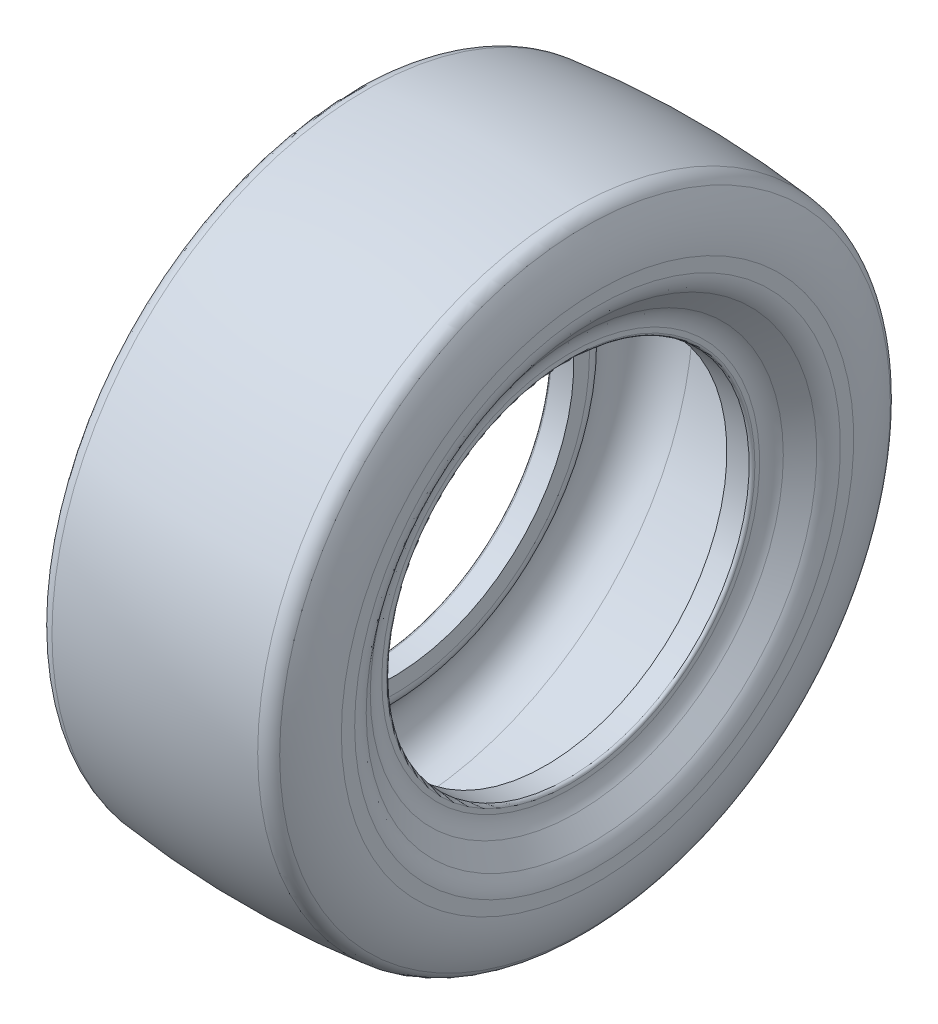
from build123d import *


with BuildPart() as part:
    # 草图1 → 旋转1 (revolve)
    with BuildSketch(Plane.XY, mode=Mode.PRIVATE) as revolve_1_sk:
        with BuildLine():
            Line((-173, 317.5), (173, 317.5))
            ThreePointArc((173, 317.5), (176.535533906, 318.964466094), (178, 322.5))
            Line((178, 322.5), (178, 330.728274474))
            ThreePointArc((178, 330.728274474), (180.73829481, 347.047932024), (188.653248902, 361.580068231))
            Line((188.653248902, 361.580068231), (214.346751098, 394.348206243))
            ThreePointArc((214.346751098, 394.348206243), (222.26170519, 408.88034245), (225, 425.2))
            Line((225, 425.2), (225, 448.5))
            ThreePointArc((225, 448.5), (219.437216248, 492.903351085), (203.092693472, 534.562188392))
            ThreePointArc((203.092693472, 534.562188392), (193.47027923, 545.122879767), (180.054342229, 550.03528168))
            ThreePointArc((180.054342229, 550.03528168), (0, 560), (-180.054342229, 550.03528168))
            ThreePointArc((-180.054342229, 550.03528168), (-193.47027923, 545.122879767), (-203.092693472, 534.562188392))
            ThreePointArc((-203.092693472, 534.562188392), (-219.437216248, 492.903351085), (-225, 448.5))
            Line((-225, 448.5), (-225, 425.2))
            ThreePointArc((-225, 425.2), (-222.26170519, 408.88034245), (-214.346751098, 394.348206243))
            Line((-214.346751098, 394.348206243), (-188.653248902, 361.580068231))
            ThreePointArc((-188.653248902, 361.580068231), (-180.73829481, 347.047932024), (-178, 330.728274474))
            Line((-178, 330.728274474), (-178, 322.5))
            ThreePointArc((-178, 322.5), (-176.535533906, 318.964466094), (-173, 317.5))
        make_face()
    revolve(revolve_1_sk.sketch.rotate(Axis((0, 0, 0), (1, 0, 0)), 90), axis=Axis((0, 0, 0), (1, 0, 0)))

    # 草图3 → 切除-旋转1 (revolve, cut)
    with BuildSketch(Plane.XY, mode=Mode.PRIVATE) as cut_revolve_1_sk:
        with BuildLine():
            Line((-134, -317.5), (134, -317.5))
            Line((134, -317.5), (134, -344.813571218))
            ThreePointArc((134, -344.813571218), (136.243708448, -356.197256004), (142.63921862, -365.878162808))
            Line((142.63921862, -365.878162808), (165.291823219, -388.84928629))
            ThreePointArc((165.291823219, -388.84928629), (180.027666262, -465.013422963), (115.45, -508))
            Line((115.45, -508), (-115.45, -508))
            ThreePointArc((-115.45, -508), (-180.027666262, -465.013422963), (-165.291823219, -388.84928629))
            Line((-165.291823219, -388.84928629), (-142.63921862, -365.878162808))
            ThreePointArc((-142.63921862, -365.878162808), (-136.243708448, -356.197256004), (-134, -344.813571218))
            Line((-134, -344.813571218), (-134, -317.5))
        make_face()
    revolve(cut_revolve_1_sk.sketch.rotate(Axis((0, 0, 0), (1, 0, 0)), 270), axis=Axis((0, 0, 0), (1, 0, 0)), mode=Mode.SUBTRACT)


solid = part.part
